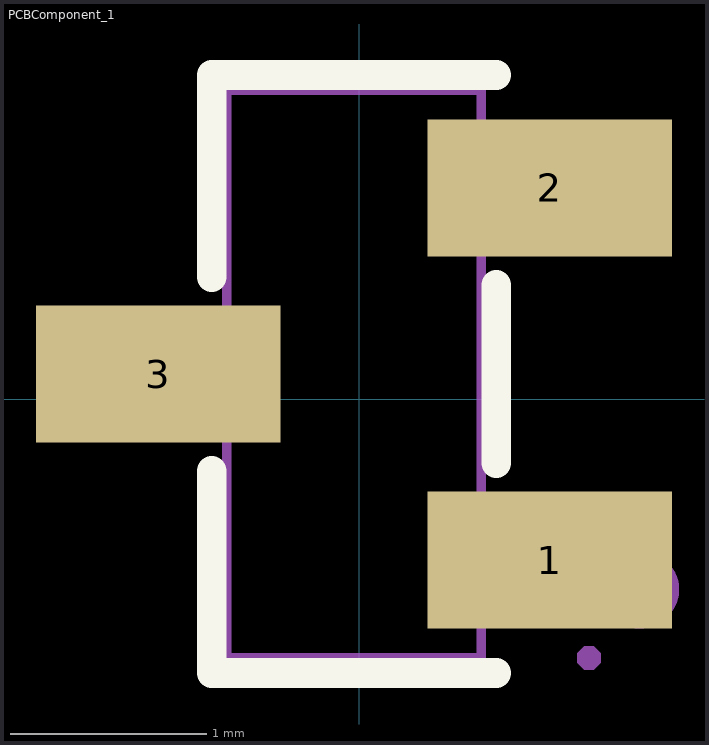
[diagram p0: the footprint, top view; thin cyan lines are the x and y axes]
# Altium footprint library MISC82341-5.PcbLib: 1 footprints
Each footprint in its own frame and in the unit in brackets; x right, y up, seen from the top. Pads: shape width x height; smd on the part's side, far side on the other; paste and mask are expansions set on the pad; w line width, h text height; cw(c..) or ccw(c..) is an arc to the next point about the centre after c.

## PCBComponent_1 [mm]
pads (3):
  rect 1.25x0.7 smd: 1(0.974,-0.821) 2(0.974,1.079) 3(-1.026,0.129)
Top Overlay:
  lines w0.152: -0.752,-0.365 -0.752,-1.397 0.7,-1.397 ; -0.752,0.624 -0.752,1.655 0.7,1.655 ; 0.7,-0.326 0.7,0.585
Mechanical 6:
  circle w0.2: c1.434,-0.971 r0.1
Mechanical 15:
  region: -1.226,-0.086 -1.226,0.344 -0.926,0.344 -0.926,-0.086
  region: -0.936,-0.086 -0.936,0.344 -0.666,0.344 -0.666,-0.086
  region: 0.874,-1.036 0.874,-0.606 1.174,-0.606 1.174,-1.036
  region: 0.614,-1.036 0.614,-0.606 0.884,-0.606 0.884,-1.036
  region: 0.874,0.864 0.874,1.294 1.174,1.294 1.174,0.864
  region: 0.614,0.864 0.614,1.294 0.884,1.294 0.884,0.864
  region: 1.234,-1.321 1.234,-1.296 1.199,-1.261 1.149,-1.261 1.114,-1.296 1.114,-1.321 1.114,-1.346 1.149,-1.381 1.199,-1.381 1.234,-1.346 1.234,-1.321
  lines w0.051: -0.676,-1.321 0.624,-1.321 0.624,1.579 -0.676,1.579 -0.676,-1.321